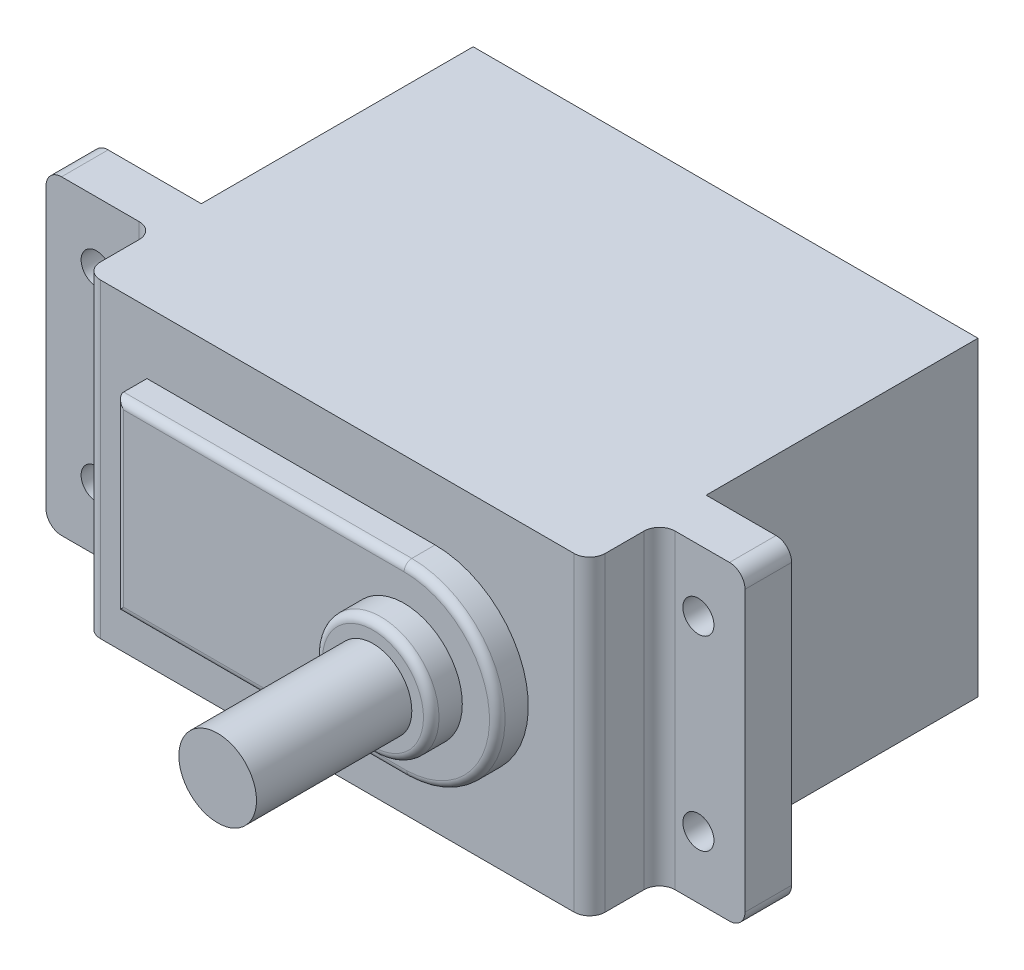
SolidWorks part; units mm, degrees
ref_plane "Front Plane" through (0, 0, 0) normal (0, 0, 1) x (1, 0, 0)
ref_plane "Top Plane" through (0, 0, 0) normal (0, 1, 0) x (1, 0, 0)
ref_plane "Right Plane" through (0, 0, 0) normal (1, 0, 0) x (0, 0, -1)
sketch "Sketch1" plane through (0, 0, 0) normal (0, 0, 1) x (1, 0, 0)
  line L1 (32.5, -20) -> (-32.5, -20)
  line L2 (32.5, -20) -> (32.5, 20)
  line L3 (32.5, 20) -> (-32.5, 20)
  line L4 (-32.5, -20) -> (-32.5, 20)
  line L5 (32.5, -20) -> (-32.5, 20) construction
  line L6 (32.5, 20) -> (-32.5, -20) construction
  point P0 (0, 0)
  dimension "D1" = 40
  dimension "D2" = 65
extrude "Boss-Extrude1" add sketch "Sketch1" along normal blind 50
sketch "Sketch2" plane through (0, 0, 50) normal (0, 0, 1) x (1, 0, 0)
  line L0 (12.6019, 12) -> (-24.5, 12)
  line L1 (-24.5, 12) -> (-24.5, -12.0001)
  line L2 (-24.5, -12.0001) -> (12.9958, -11.9935)
  line L3 (-32.5, 20) -> (-32.5, -20) construction
  arc A0 (12.2121, -11.9937) -> (12.6019, 12) centre (12.6019, 0) ccw
  dimension "D2" = 12
  dimension "D1" = 8
extrude "Boss-Extrude2" add sketch "Sketch2" along normal blind 4 contours L2 A0 L0 L1
sketch "Sketch3" plane through (0, 0, 54) normal (0, 0, 1) x (1, 0, 0)
  circle A0 centre (12.6019, 0) radius 7.5
  dimension "D1" = 15
extrude "Boss-Extrude3" add sketch "Sketch3" along normal blind 4
sketch "Sketch4" plane through (0, 0, 58) normal (0, 0, 1) x (1, 0, 0)
  circle A0 centre (12.6019, 0) radius 5
extrude "Boss-Extrude4" add sketch "Sketch4" along normal blind 20
fillet "Fillet1" radius 1 5 edges at (-5.9491, 12, 54) (-24.5, 0, 54) (-5.7521, -11.9968, 54) (24.6003, 0.197, 54) (20.1019, 0, 58)
sketch "Sketch5" plane through (32.5, 0, 0) normal (1, 0, 0) x (0, 0, -1)
  line L0 (-50, 20) -> (0, 20) construction
  line L1 (-41, 20) -> (-35, 20)
  line L2 (-41, 20) -> (-41, -20)
  line L3 (-41, -20) -> (-35, -20)
  line L4 (-35, 20) -> (-35, -20)
  line L5 (-50, -20) -> (0, -20) construction
  line L6 (-50, -20) -> (-50, 20) construction
  dimension "D1" = 15
  dimension "D2" = 6
extrude "Boss-Extrude5" add sketch "Sketch5" along normal blind 20
sketch "Sketch6" plane through (-32.5, 0, 0) normal (-1, 0, 0) x (0, 0, 1)
  line L0 (50, 20) -> (0, 20) construction
  line L1 (41, 20) -> (35, 20)
  line L2 (41, 20) -> (41, -20)
  line L3 (41, -20) -> (35, -20)
  line L4 (35, 20) -> (35, -20)
  line L5 (50, -20) -> (0, -20) construction
  line L6 (50, 20) -> (50, -20) construction
  dimension "D1" = 15
  dimension "D2" = 6
extrude "Boss-Extrude6" add sketch "Sketch6" along normal blind 20
sketch "Sketch7" plane through (0, 0, 41) normal (0, 0, 1) x (1, 0, 0)
  line L0 (-32.5, -20) -> (-32.5, 20) construction
  line L1 (-52.5, -20) -> (-32.5, -20) construction
  line L2 (-32.5, 20) -> (-32.5, -20) construction
  line L3 (-52.5, 20) -> (-32.5, 20) construction
  line L4 (52.5, 20) -> (32.5, 20) construction
  line L6 (32.5, 20) -> (32.5, -20) construction
  line L7 (52.5, -20) -> (32.5, -20) construction
  line L9 (52.5, -20) -> (43.5, -20)
  line L10 (52.5, -20) -> (52.5, 20)
  line L11 (52.5, 20) -> (43.5, 20)
  line L12 (43.5, -20) -> (43.5, 20)
  line L13 (-52.5, -20) -> (-46.5, -20)
  line L14 (-52.5, -20) -> (-52.5, 20)
  line L15 (-52.5, 20) -> (-46.5, 20)
  line L16 (-46.5, -20) -> (-46.5, 20)
  circle A0 centre (-39.98, 12) radius 2
  circle A1 centre (-39.98, -12) radius 2
  circle A2 centre (37.5, 12) radius 2
  circle A3 centre (37.5, -12) radius 2
  dimension "D1" = 4
  dimension "D2" = 4
  dimension "D3" = 4
  dimension "D4" = 4
  dimension "D11" = 5
  dimension "D12" = 8
  dimension "D5" = 7.48
  dimension "D6" = 8
  dimension "D7" = 7.48
  dimension "D8" = 8
  dimension "D9" = 8
  dimension "D10" = 5
  dimension "D13" = 6
  dimension "D14" = 9
extrude "Cut-Extrude1" cut sketch "Sketch7" against normal blind 20
fillet "Fillet2" radius 2 8 edges at (-32.5, 0, 41) (32.5, 0, 41) (32.5, 0, 50) (-32.5, 0, 50) (43.5, 20, 38) (43.5, -20, 38) (-46.5, 20, 38) (-46.5, -20, 38)
scale "Scale1" scale about origin uniform scaling yes scale factor 0.5
